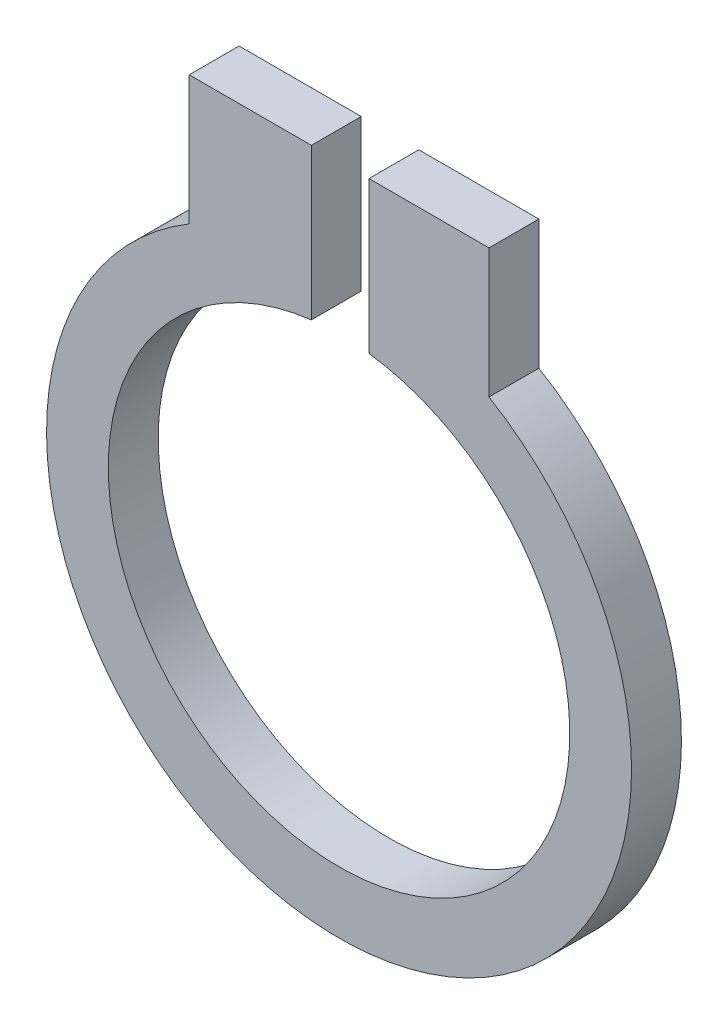
SolidWorks part; units mm, degrees
ref_plane "Front Plane" through (0, 0, 0) normal (0, 0, 1) x (1, 0, 0)
ref_plane "Top Plane" through (0, 0, 0) normal (0, 1, 0) x (1, 0, 0)
ref_plane "Right Plane" through (0, 0, 0) normal (1, 0, 0) x (0, 0, -1)
sketch "Sketch1" plane through (0, 0, 0) normal (0, 0, 1) x (1, 0, 0)
  line L0 (-0.4442, 3.6732) -> (-0.4442, 6.0978)
  line L1 (-0.4442, 6.0978) -> (-2.4024, 6.0978)
  line L2 (-2.4024, 6.0978) -> (-2.4024, 4.028)
  line L3 (0.4791, 3.6689) -> (0.4791, 6.0978)
  line L4 (0.4791, 6.0978) -> (2.404, 6.0978)
  line L5 (2.404, 6.0978) -> (2.404, 4.027)
  arc A0 (-2.4024, 4.028) -> (2.404, 4.027) centre (0, 0) ccw
  arc A1 (-0.4442, 3.6732) -> (0.4791, 3.6689) centre (0, 0) ccw
  dimension "D1" = 7.4
  dimension "D2" = 9.38
extrude "Boss-Extrude1" add sketch "Sketch1" along normal blind 0.8
